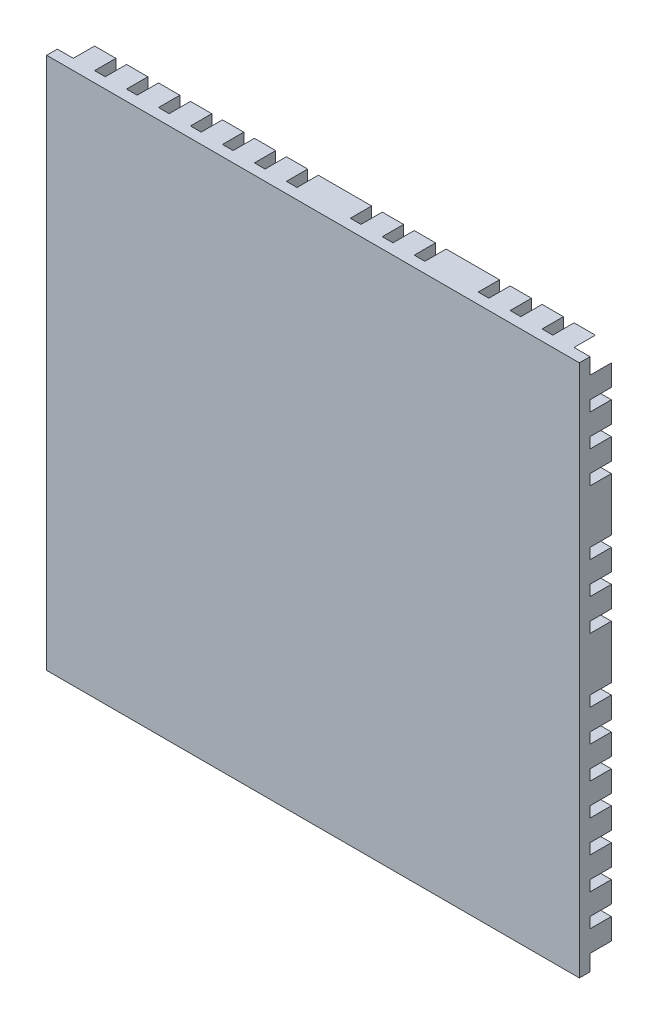
SolidWorks part; units mm, degrees
ref_plane "Front Plane" through (0, 0, 0) normal (0, 0, 1) x (1, 0, 0)
ref_plane "Top Plane" through (0, 0, 0) normal (0, 1, 0) x (1, 0, 0)
ref_plane "Right Plane" through (0, 0, 0) normal (1, 0, 0) x (0, 0, -1)
other "Configuration Table"
sketch "Sketch1" plane through (0, 0, 0) normal (0, 0, 1) x (1, 0, 0)
  line L0 (-25, 0) -> (25, 0) construction
  line L1 (-25, -25) -> (-23.5, -25)
  line L2 (-25, -25) -> (-25, -23.5)
  line L3 (-25, 25) -> (-23.5, 25)
  line L4 (25, -25) -> (25, -23.5)
  line L5 (-25, -25) -> (25, 25) construction
  line L6 (-25, 25) -> (25, -25) construction
  line L7 (0, 25) -> (0, -25) construction
  line L8 (-25, 23.5) -> (-23, 21.5)
  line L9 (-23.5, 25) -> (-21.5, 23)
  line L10 (-23.5, -25) -> (-21.5, -23)
  line L11 (-25, -23.5) -> (-23, -21.5)
  line L12 (-25, 23.5) -> (-25, 25)
  line L13 (23.5, -25) -> (25, -25)
  line L14 (25, 23.5) -> (25, 25)
  line L15 (23.5, 25) -> (25, 25)
  line L16 (-23, 21.5) -> (-25, 21.5)
  line L17 (-25, 21.5) -> (-25, 20.5)
  line L18 (-25, 20.5) -> (-22, 20.5)
  line L19 (-20, 18.5) -> (-25, 18.5)
  line L20 (-25, 18.5) -> (-25, 17.5)
  line L21 (-25, 17.5) -> (-19, 17.5)
  line L22 (-17, 15.5) -> (-25, 15.5)
  line L23 (-25, 15.5) -> (-25, 14.5)
  line L24 (-25, 14.5) -> (-16, 14.5)
  line L25 (-14, 12.5) -> (-25, 12.5)
  line L26 (-25, 12.5) -> (-25, 11.5)
  line L27 (-25, 11.5) -> (-13, 11.5)
  line L28 (-11, 9.5) -> (-25, 9.5)
  line L29 (-25, 9.5) -> (-25, 8.5)
  line L30 (-25, 8.5) -> (-10, 8.5)
  line L31 (-8, 6.5) -> (-25, 6.5)
  line L32 (-25, 6.5) -> (-25, 5.5)
  line L33 (-25, 5.5) -> (-7, 5.5)
  line L34 (-5, 3.5) -> (-25, 3.5)
  line L35 (-25, 3.5) -> (-25, 2.5)
  line L36 (-25, 2.5) -> (-4, 2.5)
  line L37 (-25, -2.5) -> (-4, -2.5)
  line L38 (-25, -3.5) -> (-25, -2.5)
  line L39 (-5, -3.5) -> (-25, -3.5)
  line L40 (-25, -5.5) -> (-7, -5.5)
  line L41 (-25, -6.5) -> (-25, -5.5)
  line L42 (-8, -6.5) -> (-25, -6.5)
  line L43 (-25, -8.5) -> (-10, -8.5)
  line L44 (-25, -9.5) -> (-25, -8.5)
  line L45 (-11, -9.5) -> (-25, -9.5)
  line L46 (-25, -11.5) -> (-13, -11.5)
  line L47 (-25, -12.5) -> (-25, -11.5)
  line L48 (-14, -12.5) -> (-25, -12.5)
  line L49 (-25, -14.5) -> (-16, -14.5)
  line L50 (-25, -15.5) -> (-25, -14.5)
  line L51 (-17, -15.5) -> (-25, -15.5)
  line L52 (-25, -17.5) -> (-19, -17.5)
  line L53 (-25, -18.5) -> (-25, -17.5)
  line L54 (-20, -18.5) -> (-25, -18.5)
  line L55 (-25, -20.5) -> (-22, -20.5)
  line L56 (-25, -21.5) -> (-25, -20.5)
  line L57 (-23, -21.5) -> (-25, -21.5)
  line L58 (-2.5, 25) -> (-2.5, 4)
  line L59 (-3.5, 25) -> (-2.5, 25)
  line L60 (-3.5, 5) -> (-3.5, 25)
  line L61 (-5.5, 25) -> (-5.5, 7)
  line L62 (-6.5, 25) -> (-5.5, 25)
  line L63 (-6.5, 8) -> (-6.5, 25)
  line L64 (-8.5, 25) -> (-8.5, 10)
  line L65 (-9.5, 25) -> (-8.5, 25)
  line L66 (-9.5, 11) -> (-9.5, 25)
  line L67 (-11.5, 25) -> (-11.5, 13)
  line L68 (-12.5, 25) -> (-11.5, 25)
  line L69 (-12.5, 14) -> (-12.5, 25)
  line L70 (-14.5, 25) -> (-14.5, 16)
  line L71 (-15.5, 25) -> (-14.5, 25)
  line L72 (-15.5, 17) -> (-15.5, 25)
  line L73 (-17.5, 25) -> (-17.5, 19)
  line L74 (-18.5, 25) -> (-17.5, 25)
  line L75 (-18.5, 20) -> (-18.5, 25)
  line L76 (-20.5, 25) -> (-20.5, 22)
  line L77 (-21.5, 25) -> (-20.5, 25)
  line L78 (-21.5, 23) -> (-21.5, 25)
  line L79 (-21.5, -23) -> (-21.5, -25)
  line L80 (-21.5, -25) -> (-20.5, -25)
  line L81 (-20.5, -25) -> (-20.5, -22)
  line L82 (-18.5, -20) -> (-18.5, -25)
  line L83 (-18.5, -25) -> (-17.5, -25)
  line L84 (-17.5, -25) -> (-17.5, -19)
  line L85 (-15.5, -17) -> (-15.5, -25)
  line L86 (-15.5, -25) -> (-14.5, -25)
  line L87 (-14.5, -25) -> (-14.5, -16)
  line L88 (-12.5, -14) -> (-12.5, -25)
  line L89 (-12.5, -25) -> (-11.5, -25)
  line L90 (-11.5, -25) -> (-11.5, -13)
  line L91 (-9.5, -11) -> (-9.5, -25)
  line L92 (-9.5, -25) -> (-8.5, -25)
  line L93 (-8.5, -25) -> (-8.5, -10)
  line L94 (-6.5, -8) -> (-6.5, -25)
  line L95 (-6.5, -25) -> (-5.5, -25)
  line L96 (-5.5, -25) -> (-5.5, -7)
  line L97 (-3.5, -5) -> (-3.5, -25)
  line L98 (-3.5, -25) -> (-2.5, -25)
  line L99 (-2.5, -25) -> (-2.5, -4)
  line L100 (21.5, 23) -> (21.5, 25)
  line L101 (21.5, 25) -> (20.5, 25)
  line L102 (20.5, 25) -> (20.5, 22)
  line L103 (18.5, 20) -> (18.5, 25)
  line L104 (18.5, 25) -> (17.5, 25)
  line L105 (17.5, 25) -> (17.5, 19)
  line L106 (15.5, 17) -> (15.5, 25)
  line L107 (15.5, 25) -> (14.5, 25)
  line L108 (14.5, 25) -> (14.5, 16)
  line L109 (12.5, 14) -> (12.5, 25)
  line L110 (12.5, 25) -> (11.5, 25)
  line L111 (11.5, 25) -> (11.5, 13)
  line L112 (9.5, 11) -> (9.5, 25)
  line L113 (9.5, 25) -> (8.5, 25)
  line L114 (8.5, 25) -> (8.5, 10)
  line L115 (6.5, 8) -> (6.5, 25)
  line L116 (6.5, 25) -> (5.5, 25)
  line L117 (5.5, 25) -> (5.5, 7)
  line L118 (3.5, 5) -> (3.5, 25)
  line L119 (3.5, 25) -> (2.5, 25)
  line L120 (2.5, 25) -> (2.5, 4)
  line L121 (25, 2.5) -> (4, 2.5)
  line L122 (25, 3.5) -> (25, 2.5)
  line L123 (5, 3.5) -> (25, 3.5)
  line L124 (25, 5.5) -> (7, 5.5)
  line L125 (25, 6.5) -> (25, 5.5)
  line L126 (8, 6.5) -> (25, 6.5)
  line L127 (25, 8.5) -> (10, 8.5)
  line L128 (25, 9.5) -> (25, 8.5)
  line L129 (11, 9.5) -> (25, 9.5)
  line L130 (25, 11.5) -> (13, 11.5)
  line L131 (25, 12.5) -> (25, 11.5)
  line L132 (14, 12.5) -> (25, 12.5)
  line L133 (25, 14.5) -> (16, 14.5)
  line L134 (25, 15.5) -> (25, 14.5)
  line L135 (17, 15.5) -> (25, 15.5)
  line L136 (25, 17.5) -> (19, 17.5)
  line L137 (25, 18.5) -> (25, 17.5)
  line L138 (20, 18.5) -> (25, 18.5)
  line L139 (25, 20.5) -> (22, 20.5)
  line L140 (25, 21.5) -> (25, 20.5)
  line L141 (23, 21.5) -> (25, 21.5)
  line L142 (23, -21.5) -> (25, -21.5)
  line L143 (25, -21.5) -> (25, -20.5)
  line L144 (25, -20.5) -> (22, -20.5)
  line L145 (20, -18.5) -> (25, -18.5)
  line L146 (25, -18.5) -> (25, -17.5)
  line L147 (25, -17.5) -> (19, -17.5)
  line L148 (17, -15.5) -> (25, -15.5)
  line L149 (25, -15.5) -> (25, -14.5)
  line L150 (25, -14.5) -> (16, -14.5)
  line L151 (14, -12.5) -> (25, -12.5)
  line L152 (25, -12.5) -> (25, -11.5)
  line L153 (25, -11.5) -> (13, -11.5)
  line L154 (11, -9.5) -> (25, -9.5)
  line L155 (25, -9.5) -> (25, -8.5)
  line L156 (25, -8.5) -> (10, -8.5)
  line L157 (8, -6.5) -> (25, -6.5)
  line L158 (25, -6.5) -> (25, -5.5)
  line L159 (25, -5.5) -> (7, -5.5)
  line L160 (5, -3.5) -> (25, -3.5)
  line L161 (25, -3.5) -> (25, -2.5)
  line L162 (25, -2.5) -> (4, -2.5)
  line L163 (2.5, -25) -> (2.5, -4)
  line L164 (3.5, -25) -> (2.5, -25)
  line L165 (3.5, -5) -> (3.5, -25)
  line L166 (5.5, -25) -> (5.5, -7)
  line L167 (6.5, -25) -> (5.5, -25)
  line L168 (6.5, -8) -> (6.5, -25)
  line L169 (8.5, -25) -> (8.5, -10)
  line L170 (9.5, -25) -> (8.5, -25)
  line L171 (9.5, -11) -> (9.5, -25)
  line L172 (11.5, -25) -> (11.5, -13)
  line L173 (12.5, -25) -> (11.5, -25)
  line L174 (12.5, -14) -> (12.5, -25)
  line L175 (14.5, -25) -> (14.5, -16)
  line L176 (15.5, -25) -> (14.5, -25)
  line L177 (15.5, -17) -> (15.5, -25)
  line L178 (17.5, -25) -> (17.5, -19)
  line L179 (18.5, -25) -> (17.5, -25)
  line L180 (18.5, -20) -> (18.5, -25)
  line L181 (20.5, -25) -> (20.5, -22)
  line L182 (21.5, -25) -> (20.5, -25)
  line L183 (21.5, -23) -> (21.5, -25)
  line L184 (1.5, 0) -> (4, -2.5)
  line L185 (0, 1.5) -> (2.5, 4)
  line L186 (0, -1.5) -> (2.5, -4)
  line L187 (1.5, 0) -> (4, 2.5)
  line L188 (-22, 20.5) -> (-20, 18.5)
  line L189 (-20.5, 22) -> (-18.5, 20)
  line L190 (-17.5, 19) -> (-15.5, 17)
  line L191 (-19, 17.5) -> (-17, 15.5)
  line L192 (-14.5, 16) -> (-12.5, 14)
  line L193 (-16, 14.5) -> (-14, 12.5)
  line L194 (-11.5, 13) -> (-9.5, 11)
  line L195 (-13, 11.5) -> (-11, 9.5)
  line L196 (-8.5, 10) -> (-6.5, 8)
  line L197 (-10, 8.5) -> (-8, 6.5)
  line L198 (-5.5, 7) -> (-3.5, 5)
  line L199 (-7, 5.5) -> (-5, 3.5)
  line L200 (-4, 2.5) -> (-1.5, 0)
  line L201 (-2.5, 4) -> (0, 1.5)
  line L202 (3.5, 5) -> (5.5, 7)
  line L203 (5, 3.5) -> (7, 5.5)
  line L204 (8, 6.5) -> (10, 8.5)
  line L205 (6.5, 8) -> (8.5, 10)
  line L206 (9.5, 11) -> (14.5, 16)
  line L207 (11, 9.5) -> (16, 14.5)
  line L208 (17, 15.5) -> (19, 17.5)
  line L209 (15.5, 17) -> (17.5, 19)
  line L210 (18.5, 20) -> (20.5, 22)
  line L211 (20, 18.5) -> (22, 20.5)
  line L212 (23, 21.5) -> (25, 23.5)
  line L213 (21.5, 23) -> (23.5, 25)
  line L214 (5, -3.5) -> (7, -5.5)
  line L215 (3.5, -5) -> (5.5, -7)
  line L216 (6.5, -8) -> (8.5, -10)
  line L217 (8, -6.5) -> (10, -8.5)
  line L218 (11, -9.5) -> (13, -11.5)
  line L219 (9.5, -11) -> (11.5, -13)
  line L220 (12.5, -14) -> (14.5, -16)
  line L221 (14, -12.5) -> (16, -14.5)
  line L222 (17, -15.5) -> (19, -17.5)
  line L223 (15.5, -17) -> (17.5, -19)
  line L224 (20, -18.5) -> (22, -20.5)
  line L225 (18.5, -20) -> (20.5, -22)
  line L226 (23, -21.5) -> (25, -23.5)
  line L227 (21.5, -23) -> (23.5, -25)
  line L228 (-2.5, -4) -> (0, -1.5)
  line L229 (-4, -2.5) -> (-1.5, 0)
  line L230 (-5.5, -7) -> (-3.5, -5)
  line L231 (-7, -5.5) -> (-5, -3.5)
  line L232 (-10, -8.5) -> (-8, -6.5)
  line L233 (-8.5, -10) -> (-6.5, -8)
  line L234 (-11.5, -13) -> (-9.5, -11)
  line L235 (-16, -14.5) -> (-14, -12.5)
  line L236 (-13, -11.5) -> (-11, -9.5)
  line L237 (-14.5, -16) -> (-12.5, -14)
  line L238 (-17.5, -19) -> (-15.5, -17)
  line L239 (-19, -17.5) -> (-17, -15.5)
  line L240 (-22, -20.5) -> (-20, -18.5)
  line L241 (-20.5, -22) -> (-18.5, -20)
  line L243 (25, -25) -> (-25, -25)
  line L244 (25, -25) -> (25, 25)
  line L245 (25, 25) -> (-25, 25)
  line L246 (-25, -25) -> (-25, 25)
  line L247 (25, -25) -> (-25, 25) construction
  line L248 (25, 25) -> (-25, -25) construction
  point P0 (0, 0)
  point P5 (0, 0)
  dimension "D7" = 2
  dimension "D8" = 1
  dimension "D9" = 25
  dimension "D10" = 2
  dimension "D11" = 1
  dimension "D12" = 2
  dimension "D13" = 1
  dimension "D14" = 2
  dimension "D15" = 1
  dimension "D16" = 2
  dimension "D17" = 1
  dimension "D18" = 2
  dimension "D19" = 1
  dimension "D20" = 2
  dimension "D21" = 1
extrude "Boss-Extrude3" add sketch "Sketch1" along normal blind 1 contours L81 L241 L82 L83 L84 L238 L85 L86 L87 L237 L88 L89 L90 L234 L91 L92 L93 L233 L94 L95 L96 L230 L97 L98 L99 L228 L186 L163 L164 L165 L215 L166 L167 L168 L216 L169 L170 L171 L219 L172 L173 L174 L220 L175 L176 L177 L223 L178 L179 L180 L225
sketch "Sketch2" plane through (0, 0, 1) normal (0, 0, 1) x (1, 0, 0)
  line L1 (25, -25) -> (-25, -25)
  line L2 (25, -25) -> (25, 25)
  line L3 (25, 25) -> (-25, 25)
  line L4 (-25, -25) -> (-25, 25)
  line L5 (25, -25) -> (-25, 25) construction
  line L6 (25, 25) -> (-25, -25) construction
  point P0 (0, 0)
extrude "Boss-Extrude4" add sketch "Sketch2" along normal blind 3 separate body
sketch "Sketch3" plane through (0, 0, 0) normal (0, 0, -1) x (-1, 0, 0)
  line L232 (20.5, -22) -> (20.5, -25)
  line L233 (20.5, -25) -> (21.5, -25)
  line L234 (21.5, -25) -> (21.5, -23)
  line L235 (21.5, -23) -> (23.5, -25)
  line L236 (23.5, -25) -> (25, -25)
  line L237 (25, -25) -> (25, -23.5)
  line L238 (25, -23.5) -> (23, -21.5)
  line L239 (23, -21.5) -> (25, -21.5)
  line L240 (25, -21.5) -> (25, -20.5)
  line L241 (25, -20.5) -> (22, -20.5)
  line L242 (22, -20.5) -> (20, -18.5)
  line L243 (20, -18.5) -> (25, -18.5)
  line L244 (25, -18.5) -> (25, -17.5)
  line L245 (25, -17.5) -> (19, -17.5)
  line L246 (19, -17.5) -> (17, -15.5)
  line L247 (17, -15.5) -> (25, -15.5)
  line L248 (25, -15.5) -> (25, -14.5)
  line L249 (25, -14.5) -> (16, -14.5)
  line L250 (16, -14.5) -> (14, -12.5)
  line L251 (14, -12.5) -> (25, -12.5)
  line L252 (25, -12.5) -> (25, -11.5)
  line L253 (25, -11.5) -> (13, -11.5)
  line L254 (13, -11.5) -> (11, -9.5)
  line L255 (11, -9.5) -> (25, -9.5)
  line L256 (25, -9.5) -> (25, -8.5)
  line L257 (25, -8.5) -> (10, -8.5)
  line L258 (10, -8.5) -> (8, -6.5)
  line L259 (8, -6.5) -> (25, -6.5)
  line L260 (25, -6.5) -> (25, -5.5)
  line L261 (25, -5.5) -> (7, -5.5)
  line L262 (7, -5.5) -> (5, -3.5)
  line L263 (5, -3.5) -> (25, -3.5)
  line L264 (25, -3.5) -> (25, -2.5)
  line L265 (25, -2.5) -> (4, -2.5)
  line L266 (4, -2.5) -> (1.5, 0)
  line L267 (1.5, 0) -> (4, 2.5)
  line L268 (4, 2.5) -> (25, 2.5)
  line L269 (25, 2.5) -> (25, 3.5)
  line L270 (25, 3.5) -> (5, 3.5)
  line L271 (5, 3.5) -> (7, 5.5)
  line L272 (7, 5.5) -> (25, 5.5)
  line L273 (25, 5.5) -> (25, 6.5)
  line L274 (25, 6.5) -> (8, 6.5)
  line L275 (8, 6.5) -> (10, 8.5)
  line L276 (10, 8.5) -> (25, 8.5)
  line L277 (25, 8.5) -> (25, 9.5)
  line L278 (25, 9.5) -> (11, 9.5)
  line L279 (11, 9.5) -> (13, 11.5)
  line L280 (13, 11.5) -> (25, 11.5)
  line L281 (25, 11.5) -> (25, 12.5)
  line L282 (25, 12.5) -> (14, 12.5)
  line L283 (14, 12.5) -> (16, 14.5)
  line L284 (16, 14.5) -> (25, 14.5)
  line L285 (25, 14.5) -> (25, 15.5)
  line L286 (25, 15.5) -> (17, 15.5)
  line L287 (17, 15.5) -> (19, 17.5)
  line L288 (19, 17.5) -> (25, 17.5)
  line L289 (25, 17.5) -> (25, 18.5)
  line L290 (25, 18.5) -> (20, 18.5)
  line L291 (20, 18.5) -> (22, 20.5)
  line L292 (22, 20.5) -> (25, 20.5)
  line L293 (25, 20.5) -> (25, 21.5)
  line L294 (25, 21.5) -> (23, 21.5)
  line L295 (23, 21.5) -> (25, 23.5)
  line L296 (25, 23.5) -> (25, 25)
  line L297 (25, 25) -> (23.5, 25)
  line L298 (23.5, 25) -> (21.5, 23)
  line L299 (21.5, 23) -> (21.5, 25)
  line L300 (21.5, 25) -> (20.5, 25)
  line L301 (20.5, 25) -> (20.5, 22)
  line L302 (20.5, 22) -> (18.5, 20)
  line L303 (18.5, 20) -> (18.5, 25)
  line L304 (18.5, 25) -> (17.5, 25)
  line L305 (17.5, 25) -> (17.5, 19)
  line L306 (17.5, 19) -> (15.5, 17)
  line L307 (15.5, 17) -> (15.5, 25)
  line L308 (15.5, 25) -> (14.5, 25)
  line L309 (14.5, 25) -> (14.5, 16)
  line L310 (14.5, 16) -> (12.5, 14)
  line L311 (12.5, 14) -> (12.5, 25)
  line L312 (12.5, 25) -> (11.5, 25)
  line L313 (11.5, 25) -> (11.5, 13)
  line L314 (11.5, 13) -> (9.5, 11)
  line L315 (9.5, 11) -> (9.5, 25)
  line L316 (9.5, 25) -> (8.5, 25)
  line L317 (8.5, 25) -> (8.5, 10)
  line L318 (8.5, 10) -> (6.5, 8)
  line L319 (6.5, 8) -> (6.5, 25)
  line L320 (6.5, 25) -> (5.5, 25)
  line L321 (5.5, 25) -> (5.5, 7)
  line L322 (5.5, 7) -> (3.5, 5)
  line L323 (3.5, 5) -> (3.5, 25)
  line L324 (3.5, 25) -> (2.5, 25)
  line L325 (2.5, 25) -> (2.5, 4)
  line L326 (2.5, 4) -> (0, 1.5)
  line L327 (0, 1.5) -> (-2.5, 4)
  line L328 (-2.5, 4) -> (-2.5, 25)
  line L329 (-2.5, 25) -> (-3.5, 25)
  line L330 (-3.5, 25) -> (-3.5, 5)
  line L331 (-3.5, 5) -> (-5.5, 7)
  line L332 (-5.5, 7) -> (-5.5, 25)
  line L333 (-5.5, 25) -> (-6.5, 25)
  line L334 (-6.5, 25) -> (-6.5, 8)
  line L335 (-6.5, 8) -> (-8.5, 10)
  line L336 (-8.5, 10) -> (-8.5, 25)
  line L337 (-8.5, 25) -> (-9.5, 25)
  line L338 (-9.5, 25) -> (-9.5, 11)
  line L339 (-9.5, 11) -> (-14.5, 16)
  line L340 (-14.5, 16) -> (-14.5, 25)
  line L341 (-14.5, 25) -> (-15.5, 25)
  line L342 (-15.5, 25) -> (-15.5, 17)
  line L343 (-15.5, 17) -> (-17.5, 19)
  line L344 (-17.5, 19) -> (-17.5, 25)
  line L345 (-17.5, 25) -> (-18.5, 25)
  line L346 (-18.5, 25) -> (-18.5, 20)
  line L347 (-18.5, 20) -> (-20.5, 22)
  line L348 (-20.5, 22) -> (-20.5, 25)
  line L349 (-20.5, 25) -> (-21.5, 25)
  line L350 (-21.5, 25) -> (-21.5, 23)
  line L351 (-21.5, 23) -> (-23.5, 25)
  line L352 (-23.5, 25) -> (-25, 25)
  line L353 (-25, 25) -> (-25, 23.5)
  line L354 (-25, 23.5) -> (-23, 21.5)
  line L355 (-23, 21.5) -> (-25, 21.5)
  line L356 (-25, 21.5) -> (-25, 20.5)
  line L357 (-25, 20.5) -> (-22, 20.5)
  line L358 (-22, 20.5) -> (-20, 18.5)
  line L359 (-20, 18.5) -> (-25, 18.5)
  line L360 (-25, 18.5) -> (-25, 17.5)
  line L361 (-25, 17.5) -> (-19, 17.5)
  line L362 (-19, 17.5) -> (-17, 15.5)
  line L363 (-17, 15.5) -> (-25, 15.5)
  line L364 (-25, 15.5) -> (-25, 14.5)
  line L365 (-25, 14.5) -> (-16, 14.5)
  line L366 (-16, 14.5) -> (-11, 9.5)
  line L367 (-11, 9.5) -> (-25, 9.5)
  line L368 (-25, 9.5) -> (-25, 8.5)
  line L369 (-25, 8.5) -> (-10, 8.5)
  line L370 (-10, 8.5) -> (-8, 6.5)
  line L371 (-8, 6.5) -> (-25, 6.5)
  line L372 (-25, 6.5) -> (-25, 5.5)
  line L373 (-25, 5.5) -> (-7, 5.5)
  line L374 (-7, 5.5) -> (-5, 3.5)
  line L375 (-5, 3.5) -> (-25, 3.5)
  line L376 (-25, 3.5) -> (-25, 2.5)
  line L377 (-25, 2.5) -> (-4, 2.5)
  line L378 (-4, 2.5) -> (-1.5, 0)
  line L379 (-1.5, 0) -> (-4, -2.5)
  line L380 (-4, -2.5) -> (-25, -2.5)
  line L381 (-25, -2.5) -> (-25, -3.5)
  line L382 (-25, -3.5) -> (-5, -3.5)
  line L383 (-5, -3.5) -> (-7, -5.5)
  line L384 (-7, -5.5) -> (-25, -5.5)
  line L385 (-25, -5.5) -> (-25, -6.5)
  line L386 (-25, -6.5) -> (-8, -6.5)
  line L387 (-8, -6.5) -> (-10, -8.5)
  line L388 (-10, -8.5) -> (-25, -8.5)
  line L389 (-25, -8.5) -> (-25, -9.5)
  line L390 (-25, -9.5) -> (-11, -9.5)
  line L391 (-11, -9.5) -> (-13, -11.5)
  line L392 (-13, -11.5) -> (-25, -11.5)
  line L393 (-25, -11.5) -> (-25, -12.5)
  line L394 (-25, -12.5) -> (-14, -12.5)
  line L395 (-14, -12.5) -> (-16, -14.5)
  line L396 (-16, -14.5) -> (-25, -14.5)
  line L397 (-25, -14.5) -> (-25, -15.5)
  line L398 (-25, -15.5) -> (-17, -15.5)
  line L399 (-17, -15.5) -> (-19, -17.5)
  line L400 (-19, -17.5) -> (-25, -17.5)
  line L401 (-25, -17.5) -> (-25, -18.5)
  line L402 (-25, -18.5) -> (-20, -18.5)
  line L403 (-20, -18.5) -> (-22, -20.5)
  line L404 (-22, -20.5) -> (-25, -20.5)
  line L405 (-25, -20.5) -> (-25, -21.5)
  line L406 (-25, -21.5) -> (-23, -21.5)
  line L407 (-23, -21.5) -> (-25, -23.5)
  line L408 (-25, -23.5) -> (-25, -25)
  line L409 (-25, -25) -> (-23.5, -25)
  line L410 (-23.5, -25) -> (-21.5, -23)
  line L411 (-21.5, -23) -> (-21.5, -25)
  line L412 (-21.5, -25) -> (-20.5, -25)
  line L413 (-20.5, -25) -> (-20.5, -22)
  line L414 (-20.5, -22) -> (-18.5, -20)
  line L415 (-18.5, -20) -> (-18.5, -25)
  line L416 (-18.5, -25) -> (-17.5, -25)
  line L417 (-17.5, -25) -> (-17.5, -19)
  line L418 (-17.5, -19) -> (-15.5, -17)
  line L419 (-15.5, -17) -> (-15.5, -25)
  line L420 (-15.5, -25) -> (-14.5, -25)
  line L421 (-14.5, -25) -> (-14.5, -16)
  line L422 (-14.5, -16) -> (-12.5, -14)
  line L423 (-12.5, -14) -> (-12.5, -25)
  line L424 (-12.5, -25) -> (-11.5, -25)
  line L425 (-11.5, -25) -> (-11.5, -13)
  line L426 (-11.5, -13) -> (-9.5, -11)
  line L427 (-9.5, -11) -> (-9.5, -25)
  line L428 (-9.5, -25) -> (-8.5, -25)
  line L429 (-8.5, -25) -> (-8.5, -10)
  line L430 (-8.5, -10) -> (-6.5, -8)
  line L431 (-6.5, -8) -> (-6.5, -25)
  line L432 (-6.5, -25) -> (-5.5, -25)
  line L433 (-5.5, -25) -> (-5.5, -7)
  line L434 (-5.5, -7) -> (-3.5, -5)
  line L435 (-3.5, -5) -> (-3.5, -25)
  line L436 (-3.5, -25) -> (-2.5, -25)
  line L437 (-2.5, -25) -> (-2.5, -4)
  line L438 (-2.5, -4) -> (0, -1.5)
  line L439 (0, -1.5) -> (2.5, -4)
  line L440 (2.5, -4) -> (2.5, -25)
  line L441 (2.5, -25) -> (3.5, -25)
  line L442 (3.5, -25) -> (3.5, -5)
  line L443 (3.5, -5) -> (5.5, -7)
  line L444 (5.5, -7) -> (5.5, -25)
  line L445 (5.5, -25) -> (6.5, -25)
  line L446 (6.5, -25) -> (6.5, -8)
  line L447 (6.5, -8) -> (8.5, -10)
  line L448 (8.5, -10) -> (8.5, -25)
  line L449 (8.5, -25) -> (9.5, -25)
  line L450 (9.5, -25) -> (9.5, -11)
  line L451 (9.5, -11) -> (11.5, -13)
  line L452 (11.5, -13) -> (11.5, -25)
  line L453 (11.5, -25) -> (12.5, -25)
  line L454 (12.5, -25) -> (12.5, -14)
  line L455 (12.5, -14) -> (14.5, -16)
  line L456 (14.5, -16) -> (14.5, -25)
  line L457 (14.5, -25) -> (15.5, -25)
  line L458 (15.5, -25) -> (15.5, -17)
  line L459 (15.5, -17) -> (17.5, -19)
  line L460 (17.5, -19) -> (17.5, -25)
  line L461 (17.5, -25) -> (18.5, -25)
  line L462 (18.5, -25) -> (18.5, -20)
  line L463 (18.5, -20) -> (20.5, -22)
  line L464 (20.5, -22) -> (20.5, -25)
  line L465 (20.5, -25) -> (21.5, -25)
  line L466 (21.5, -25) -> (21.5, -23)
  line L467 (21.5, -23) -> (23.5, -25)
  line L468 (23.5, -25) -> (25, -25)
  line L469 (25, -25) -> (25, -23.5)
  line L470 (25, -23.5) -> (23, -21.5)
  line L471 (23, -21.5) -> (25, -21.5)
  line L472 (25, -21.5) -> (25, -20.5)
  line L473 (25, -20.5) -> (22, -20.5)
  line L474 (22, -20.5) -> (20, -18.5)
  line L475 (20, -18.5) -> (25, -18.5)
  line L476 (25, -18.5) -> (25, -17.5)
  line L477 (25, -17.5) -> (19, -17.5)
  line L478 (19, -17.5) -> (17, -15.5)
  line L479 (17, -15.5) -> (25, -15.5)
  line L480 (25, -15.5) -> (25, -14.5)
  line L481 (25, -14.5) -> (16, -14.5)
  line L482 (16, -14.5) -> (14, -12.5)
  line L483 (14, -12.5) -> (25, -12.5)
  line L484 (25, -12.5) -> (25, -11.5)
  line L485 (25, -11.5) -> (13, -11.5)
  line L486 (13, -11.5) -> (11, -9.5)
  line L487 (11, -9.5) -> (25, -9.5)
  line L488 (25, -9.5) -> (25, -8.5)
  line L489 (25, -8.5) -> (10, -8.5)
  line L490 (10, -8.5) -> (8, -6.5)
  line L491 (8, -6.5) -> (25, -6.5)
  line L492 (25, -6.5) -> (25, -5.5)
  line L493 (25, -5.5) -> (7, -5.5)
  line L494 (7, -5.5) -> (5, -3.5)
  line L495 (5, -3.5) -> (25, -3.5)
  line L496 (25, -3.5) -> (25, -2.5)
  line L497 (25, -2.5) -> (4, -2.5)
  line L498 (4, -2.5) -> (1.5, 0)
  line L499 (1.5, 0) -> (4, 2.5)
  line L500 (4, 2.5) -> (25, 2.5)
  line L501 (25, 2.5) -> (25, 3.5)
  line L502 (25, 3.5) -> (5, 3.5)
  line L503 (5, 3.5) -> (7, 5.5)
  line L504 (7, 5.5) -> (25, 5.5)
  line L505 (25, 5.5) -> (25, 6.5)
  line L506 (25, 6.5) -> (8, 6.5)
  line L507 (8, 6.5) -> (10, 8.5)
  line L508 (10, 8.5) -> (25, 8.5)
  line L509 (25, 8.5) -> (25, 9.5)
  line L510 (25, 9.5) -> (11, 9.5)
  line L511 (11, 9.5) -> (13, 11.5)
  line L512 (13, 11.5) -> (25, 11.5)
  line L513 (25, 11.5) -> (25, 12.5)
  line L514 (25, 12.5) -> (14, 12.5)
  line L515 (14, 12.5) -> (16, 14.5)
  line L516 (16, 14.5) -> (25, 14.5)
  line L517 (25, 14.5) -> (25, 15.5)
  line L518 (25, 15.5) -> (17, 15.5)
  line L519 (17, 15.5) -> (19, 17.5)
  line L520 (19, 17.5) -> (25, 17.5)
  line L521 (25, 17.5) -> (25, 18.5)
  line L522 (25, 18.5) -> (20, 18.5)
  line L523 (20, 18.5) -> (22, 20.5)
  line L524 (22, 20.5) -> (25, 20.5)
  line L525 (25, 20.5) -> (25, 21.5)
  line L526 (25, 21.5) -> (23, 21.5)
  line L527 (23, 21.5) -> (25, 23.5)
  line L528 (25, 23.5) -> (25, 25)
  line L529 (25, 25) -> (23.5, 25)
  line L530 (23.5, 25) -> (21.5, 23)
  line L531 (21.5, 23) -> (21.5, 25)
  line L532 (21.5, 25) -> (20.5, 25)
  line L533 (20.5, 25) -> (20.5, 22)
  line L534 (20.5, 22) -> (18.5, 20)
  line L535 (18.5, 20) -> (18.5, 25)
  line L536 (18.5, 25) -> (17.5, 25)
  line L537 (17.5, 25) -> (17.5, 19)
  line L538 (17.5, 19) -> (15.5, 17)
  line L539 (15.5, 17) -> (15.5, 25)
  line L540 (15.5, 25) -> (14.5, 25)
  line L541 (14.5, 25) -> (14.5, 16)
  line L542 (14.5, 16) -> (12.5, 14)
  line L543 (12.5, 14) -> (12.5, 25)
  line L544 (12.5, 25) -> (11.5, 25)
  line L545 (11.5, 25) -> (11.5, 13)
  line L546 (11.5, 13) -> (9.5, 11)
  line L547 (9.5, 11) -> (9.5, 25)
  line L548 (9.5, 25) -> (8.5, 25)
  line L549 (8.5, 25) -> (8.5, 10)
  line L550 (8.5, 10) -> (6.5, 8)
  line L551 (6.5, 8) -> (6.5, 25)
  line L552 (6.5, 25) -> (5.5, 25)
  line L553 (5.5, 25) -> (5.5, 7)
  line L554 (5.5, 7) -> (3.5, 5)
  line L555 (3.5, 5) -> (3.5, 25)
  line L556 (3.5, 25) -> (2.5, 25)
  line L557 (2.5, 25) -> (2.5, 4)
  line L558 (2.5, 4) -> (0, 1.5)
  line L559 (0, 1.5) -> (-2.5, 4)
  line L560 (-2.5, 4) -> (-2.5, 25)
  line L561 (-2.5, 25) -> (-3.5, 25)
  line L562 (-3.5, 25) -> (-3.5, 5)
  line L563 (-3.5, 5) -> (-5.5, 7)
  line L564 (-5.5, 7) -> (-5.5, 25)
  line L565 (-5.5, 25) -> (-6.5, 25)
  line L566 (-6.5, 25) -> (-6.5, 8)
  line L567 (-6.5, 8) -> (-8.5, 10)
  line L568 (-8.5, 10) -> (-8.5, 25)
  line L569 (-8.5, 25) -> (-9.5, 25)
  line L570 (-9.5, 25) -> (-9.5, 11)
  line L571 (-9.5, 11) -> (-14.5, 16)
  line L572 (-14.5, 16) -> (-14.5, 25)
  line L573 (-14.5, 25) -> (-15.5, 25)
  line L574 (-15.5, 25) -> (-15.5, 17)
  line L575 (-15.5, 17) -> (-17.5, 19)
  line L576 (-17.5, 19) -> (-17.5, 25)
  line L577 (-17.5, 25) -> (-18.5, 25)
  line L578 (-18.5, 25) -> (-18.5, 20)
  line L579 (-18.5, 20) -> (-20.5, 22)
  line L580 (-20.5, 22) -> (-20.5, 25)
  line L581 (-20.5, 25) -> (-21.5, 25)
  line L582 (-21.5, 25) -> (-21.5, 23)
  line L583 (-21.5, 23) -> (-23.5, 25)
  line L584 (-23.5, 25) -> (-25, 25)
  line L585 (-25, 25) -> (-25, 23.5)
  line L586 (-25, 23.5) -> (-23, 21.5)
  line L587 (-23, 21.5) -> (-25, 21.5)
  line L588 (-25, 21.5) -> (-25, 20.5)
  line L589 (-25, 20.5) -> (-22, 20.5)
  line L590 (-22, 20.5) -> (-20, 18.5)
  line L591 (-20, 18.5) -> (-25, 18.5)
  line L592 (-25, 18.5) -> (-25, 17.5)
  line L593 (-25, 17.5) -> (-19, 17.5)
  line L594 (-19, 17.5) -> (-17, 15.5)
  line L595 (-17, 15.5) -> (-25, 15.5)
  line L596 (-25, 15.5) -> (-25, 14.5)
  line L597 (-25, 14.5) -> (-16, 14.5)
  line L598 (-16, 14.5) -> (-11, 9.5)
  line L599 (-11, 9.5) -> (-25, 9.5)
  line L600 (-25, 9.5) -> (-25, 8.5)
  line L601 (-25, 8.5) -> (-10, 8.5)
  line L602 (-10, 8.5) -> (-8, 6.5)
  line L603 (-8, 6.5) -> (-25, 6.5)
  line L604 (-25, 6.5) -> (-25, 5.5)
  line L605 (-25, 5.5) -> (-7, 5.5)
  line L606 (-7, 5.5) -> (-5, 3.5)
  line L607 (-5, 3.5) -> (-25, 3.5)
  line L608 (-25, 3.5) -> (-25, 2.5)
  line L609 (-25, 2.5) -> (-4, 2.5)
  line L610 (-4, 2.5) -> (-1.5, 0)
  line L611 (-1.5, 0) -> (-4, -2.5)
  line L612 (-4, -2.5) -> (-25, -2.5)
  line L613 (-25, -2.5) -> (-25, -3.5)
  line L614 (-25, -3.5) -> (-5, -3.5)
  line L615 (-5, -3.5) -> (-7, -5.5)
  line L616 (-7, -5.5) -> (-25, -5.5)
  line L617 (-25, -5.5) -> (-25, -6.5)
  line L618 (-25, -6.5) -> (-8, -6.5)
  line L619 (-8, -6.5) -> (-10, -8.5)
  line L620 (-10, -8.5) -> (-25, -8.5)
  line L621 (-25, -8.5) -> (-25, -9.5)
  line L622 (-25, -9.5) -> (-11, -9.5)
  line L623 (-11, -9.5) -> (-13, -11.5)
  line L624 (-13, -11.5) -> (-25, -11.5)
  line L625 (-25, -11.5) -> (-25, -12.5)
  line L626 (-25, -12.5) -> (-14, -12.5)
  line L627 (-14, -12.5) -> (-16, -14.5)
  line L628 (-16, -14.5) -> (-25, -14.5)
  line L629 (-25, -14.5) -> (-25, -15.5)
  line L630 (-25, -15.5) -> (-17, -15.5)
  line L631 (-17, -15.5) -> (-19, -17.5)
  line L632 (-19, -17.5) -> (-25, -17.5)
  line L633 (-25, -17.5) -> (-25, -18.5)
  line L634 (-25, -18.5) -> (-20, -18.5)
  line L635 (-20, -18.5) -> (-22, -20.5)
  line L636 (-22, -20.5) -> (-25, -20.5)
  line L637 (-25, -20.5) -> (-25, -21.5)
  line L638 (-25, -21.5) -> (-23, -21.5)
  line L639 (-23, -21.5) -> (-25, -23.5)
  line L640 (-25, -23.5) -> (-25, -25)
  line L641 (-25, -25) -> (-23.5, -25)
  line L642 (-23.5, -25) -> (-21.5, -23)
  line L643 (-21.5, -23) -> (-21.5, -25)
  line L644 (-21.5, -25) -> (-20.5, -25)
  line L645 (-20.5, -25) -> (-20.5, -22)
  line L646 (-20.5, -22) -> (-18.5, -20)
  line L647 (-18.5, -20) -> (-18.5, -25)
  line L648 (-18.5, -25) -> (-17.5, -25)
  line L649 (-17.5, -25) -> (-17.5, -19)
  line L650 (-17.5, -19) -> (-15.5, -17)
  line L651 (-15.5, -17) -> (-15.5, -25)
  line L652 (-15.5, -25) -> (-14.5, -25)
  line L653 (-14.5, -25) -> (-14.5, -16)
  line L654 (-14.5, -16) -> (-12.5, -14)
  line L655 (-12.5, -14) -> (-12.5, -25)
  line L656 (-12.5, -25) -> (-11.5, -25)
  line L657 (-11.5, -25) -> (-11.5, -13)
  line L658 (-11.5, -13) -> (-9.5, -11)
  line L659 (-9.5, -11) -> (-9.5, -25)
  line L660 (-9.5, -25) -> (-8.5, -25)
  line L661 (-8.5, -25) -> (-8.5, -10)
  line L662 (-8.5, -10) -> (-6.5, -8)
  line L663 (-6.5, -8) -> (-6.5, -25)
  line L664 (-6.5, -25) -> (-5.5, -25)
  line L665 (-5.5, -25) -> (-5.5, -7)
  line L666 (-5.5, -7) -> (-3.5, -5)
  line L667 (-3.5, -5) -> (-3.5, -25)
  line L668 (-3.5, -25) -> (-2.5, -25)
  line L669 (-2.5, -25) -> (-2.5, -4)
  line L670 (-2.5, -4) -> (0, -1.5)
  line L671 (0, -1.5) -> (2.5, -4)
  line L672 (2.5, -4) -> (2.5, -25)
  line L673 (2.5, -25) -> (3.5, -25)
  line L674 (3.5, -25) -> (3.5, -5)
  line L675 (3.5, -5) -> (5.5, -7)
  line L676 (5.5, -7) -> (5.5, -25)
  line L677 (5.5, -25) -> (6.5, -25)
  line L678 (6.5, -25) -> (6.5, -8)
  line L679 (6.5, -8) -> (8.5, -10)
  line L680 (8.5, -10) -> (8.5, -25)
  line L681 (8.5, -25) -> (9.5, -25)
  line L682 (9.5, -25) -> (9.5, -11)
  line L683 (9.5, -11) -> (11.5, -13)
  line L684 (11.5, -13) -> (11.5, -25)
  line L685 (11.5, -25) -> (12.5, -25)
  line L686 (12.5, -25) -> (12.5, -14)
  line L687 (12.5, -14) -> (14.5, -16)
  line L688 (14.5, -16) -> (14.5, -25)
  line L689 (14.5, -25) -> (15.5, -25)
  line L690 (15.5, -25) -> (15.5, -17)
  line L691 (15.5, -17) -> (17.5, -19)
  line L692 (17.5, -19) -> (17.5, -25)
  line L693 (17.5, -25) -> (18.5, -25)
  line L694 (18.5, -25) -> (18.5, -20)
  line L695 (18.5, -20) -> (20.5, -22)
  dimension "D1" = 0
extrude "Cut-Extrude1" cut sketch "Sketch3" against normal blind 3
